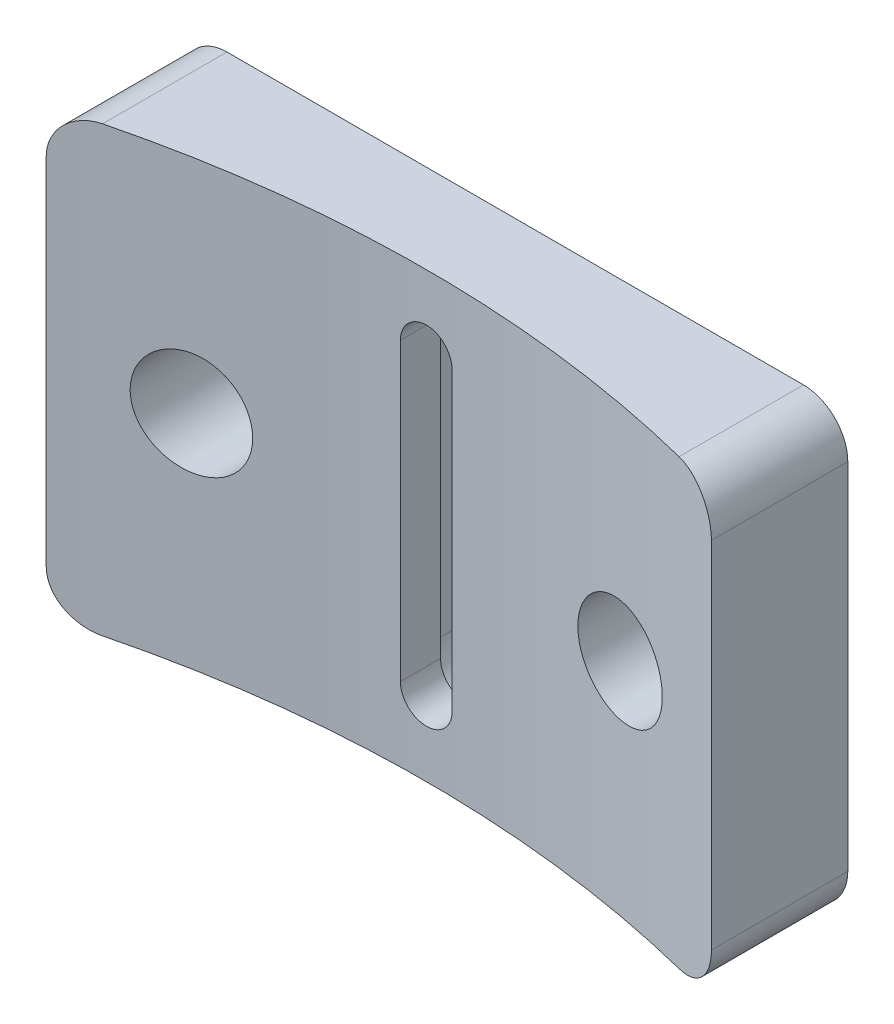
from build123d import *

# Parameters (mm, degrees)
BOSS_EXTRUDE1_DEPTH   = 30
M8X1_0_TAPPED_HOLE1_D = 7
CUT_EXTRUDE1_DEPTH    = 39.619021662
CUT_EXTRUDE2_DEPTH    = 3.3
FILLET1_R             = 3


with BuildPart() as part:
    # Sketch1 → Boss-Extrude1 (new body)
    with BuildSketch(Plane(origin=(0, 0, 0), x_dir=(1, 0, 0), z_dir=(0, 1, 0))):
        with BuildLine():
            Line((-22.5, 76.770762664), (-22.5, 86))
            Line((-22.5, 86), (22.5, 86))
            Line((22.5, 86), (22.5, 76.770762664))
            ThreePointArc((22.5, 76.770762664), (0, 80), (-22.5, 76.770762664))
        make_face()
    extrude(amount=BOSS_EXTRUDE1_DEPTH)

    # M8x1.0 Tapped Hole1 (through all)
    with Locations(Plane(origin=(0, 0, -86), x_dir=(-1, 0, 0), z_dir=(0, 0, -1))):
        with Locations((-14.5, 15), (14.5, 15)):
            Hole(M8X1_0_TAPPED_HOLE1_D / 2)

    # Sketch4 → Cut-Extrude1 (cut, through all)
    with BuildSketch(Plane(origin=(0, 0, -86), x_dir=(-1, 0, 0), z_dir=(0, 0, -1))):
        with BuildLine():
            Line((1.75, 25), (1.75, 5))
            ThreePointArc((1.75, 5), (0, 3.25), (-1.75, 5))
            Line((-1.75, 5), (-1.75, 25))
            ThreePointArc((-1.75, 25), (0, 26.75), (1.75, 25))
        make_face()
    extrude(amount=-CUT_EXTRUDE1_DEPTH, mode=Mode.SUBTRACT)

    # Sketch5 → Cut-Extrude2 (cut)
    with BuildSketch(Plane(origin=(0, 0, -86), x_dir=(-1, 0, 0), z_dir=(0, 0, -1))):
        with BuildLine():
            Line((3, 25), (3, 5))
            ThreePointArc((3, 5), (0, 2), (-3, 5))
            Line((-3, 5), (-3, 25))
            ThreePointArc((-3, 25), (0, 28), (3, 25))
        make_face()
    extrude(amount=-CUT_EXTRUDE2_DEPTH, mode=Mode.SUBTRACT)

    # Fillet1
    fillet1_edges = [part.edges().sort_by_distance(p)[0] for p in [
        (22.5, 30, -81.385381332),
        (22.5, 0, -81.385381332),
        (-22.5, 0, -81.385381332),
        (-22.5, 30, -81.385381332),
    ]]
    fillet(fillet1_edges, radius=FILLET1_R)


solid = part.part
